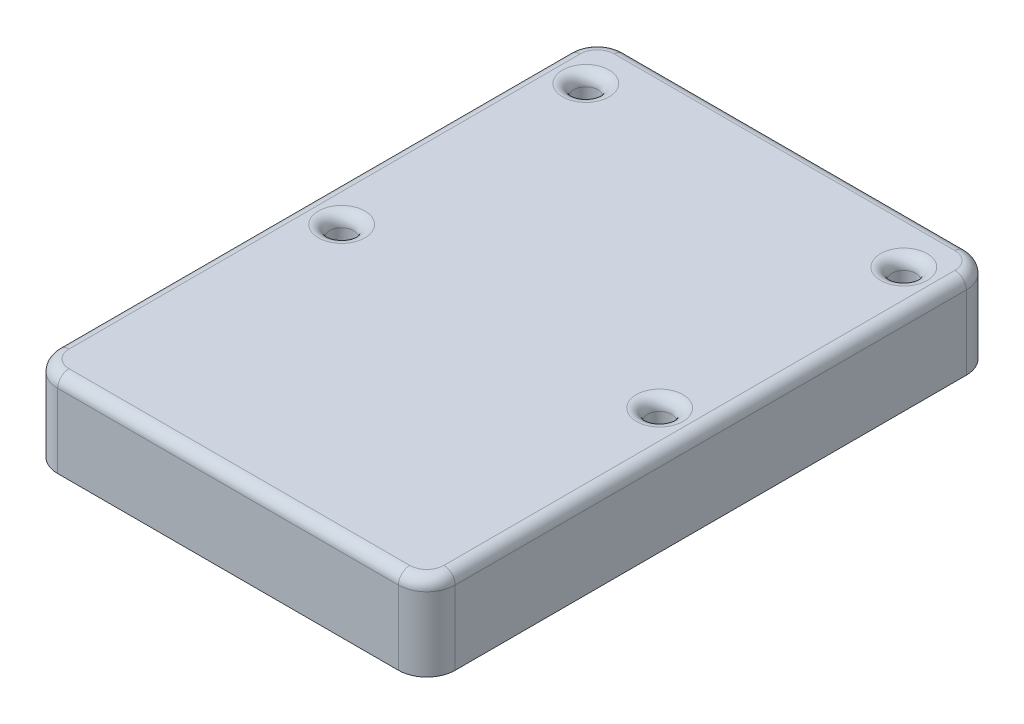
from build123d import *

# Parameters (mm, degrees)
BOSS_EXTRUDE1_DEPTH = 15
CUT_EXTRUDE1_DEPTH  = 12
CUT_EXTRUDE2_DEPTH  = 1
BOSS_EXTRUDE2_START = 11
BOSS_EXTRUDE2_DEPTH = 11
SKETCH5_R           = 1.2
CUT_EXTRUDE3_DEPTH  = 63.84902545
SKETCH6_R           = 2.1
CUT_EXTRUDE4_DEPTH  = 12
FILLET1_R           = 2
SCALE1_SCALE        = 0.5
FILLET2_R           = 1


with BuildPart() as part:
    # Sketch1 → Boss-Extrude1 (new body)
    with BuildSketch(Plane(origin=(0, 0, 0), x_dir=(1, 0, 0), z_dir=(0, 1, 0))):
        with BuildLine():
            Line((-30, -50), (30, -50))
            ThreePointArc((30, -50), (33.535533906, -48.535533906), (35, -45))
            Line((35, -45), (35, 45))
            ThreePointArc((35, 45), (33.535533906, 48.535533906), (30, 50))
            Line((30, 50), (-30, 50))
            ThreePointArc((-30, 50), (-33.535533906, 48.535533906), (-35, 45))
            Line((-35, 45), (-35, -45))
            ThreePointArc((-35, -45), (-33.535533906, -48.535533906), (-30, -50))
        make_face()
    extrude(amount=BOSS_EXTRUDE1_DEPTH)

    # Sketch2 → Cut-Extrude1 (cut)
    with BuildSketch(Plane.XZ):
        with BuildLine():
            Line((-27, -47), (27, -47))
            ThreePointArc((27, -47), (30.535533906, -45.535533906), (32, -42))
            Line((32, -42), (32, 42))
            ThreePointArc((32, 42), (30.535533906, 45.535533906), (27, 47))
            Line((27, 47), (-27, 47))
            ThreePointArc((-27, 47), (-30.535533906, 45.535533906), (-32, 42))
            Line((-32, 42), (-32, -42))
            ThreePointArc((-32, -42), (-30.535533906, -45.535533906), (-27, -47))
        make_face()
    extrude(amount=-CUT_EXTRUDE1_DEPTH, mode=Mode.SUBTRACT)

    # Sketch3 → Cut-Extrude2 (cut)
    with BuildSketch(Plane.XZ):
        with BuildLine():
            Line((-27, -48.55), (27, -48.55))
            ThreePointArc((27, -48.55), (31.631549417, -46.631549417), (33.55, -42))
            Line((33.55, -42), (33.55, 42))
            ThreePointArc((33.55, 42), (31.631549417, 46.631549417), (27, 48.55))
            Line((27, 48.55), (-27, 48.55))
            ThreePointArc((-27, 48.55), (-31.631549417, 46.631549417), (-33.55, 42))
            Line((-33.55, 42), (-33.55, -42))
            ThreePointArc((-33.55, -42), (-31.631549417, -46.631549417), (-27, -48.55))
        make_face()
        with BuildLine():
            Line((-27, -47), (27, -47))
            ThreePointArc((27, -47), (30.535533906, -45.535533906), (32, -42))
            Line((32, -42), (32, 42))
            ThreePointArc((32, 42), (30.535533906, 45.535533906), (27, 47))
            Line((27, 47), (-27, 47))
            ThreePointArc((-27, 47), (-30.535533906, 45.535533906), (-32, 42))
            Line((-32, 42), (-32, -42))
            ThreePointArc((-32, -42), (-30.535533906, -45.535533906), (-27, -47))
        make_face(mode=Mode.SUBTRACT)
    extrude(amount=-CUT_EXTRUDE2_DEPTH, mode=Mode.SUBTRACT)

    # Sketch4 → Boss-Extrude2 (add)
    with BuildSketch(Plane.XZ.offset(-12).offset(BOSS_EXTRUDE2_START)):
        with BuildLine():
            ThreePointArc((-28, -2), (-24, 2), (-28, 6))
            Line((-28, 6), (-32, 6))
            Line((-32, 6), (-32, -2))
            Line((-32, -2), (-28, -2))
        make_face()
        with BuildLine():
            Line((-28, -37), (-32, -37))
            Line((-32, -37), (-32, -42))
            ThreePointArc((-32, -42), (-30.535533906, -45.535533906), (-27, -47))
            Line((-27, -47), (-24, -47))
            Line((-24, -47), (-24, -41))
            ThreePointArc((-24, -41), (-25.171572875, -38.171572875), (-28, -37))
        make_face()
        with BuildLine():
            Line((32, -2), (32, 6))
            Line((32, 6), (28, 6))
            ThreePointArc((28, 6), (24, 2), (28, -2))
            Line((28, -2), (32, -2))
        make_face()
        with BuildLine():
            Line((24, -41), (24, -47))
            Line((24, -47), (27, -47))
            ThreePointArc((27, -47), (30.535533906, -45.535533906), (32, -42))
            Line((32, -42), (32, -37))
            Line((32, -37), (28, -37))
            ThreePointArc((28, -37), (25.171572875, -38.171572875), (24, -41))
        make_face()
    extrude(amount=-BOSS_EXTRUDE2_DEPTH)

    # Sketch5 → Cut-Extrude3 (cut, through all)
    with BuildSketch(Plane(origin=(0, 15, 0), x_dir=(1, 0, 0), z_dir=(0, 1, 0))):
        with Locations(Location((28, -2, 0), (0, 0, 270))):
            Circle(SKETCH5_R)
        with Locations(Location((28, 41, 0), (0, 0, 270))):
            Circle(SKETCH5_R)
        with Locations(Location((-28, 41, 0), (0, 0, 270))):
            Circle(SKETCH5_R)
        with Locations(Location((-28, -2, 0), (0, 0, 270))):
            Circle(SKETCH5_R)
    extrude(amount=-CUT_EXTRUDE3_DEPTH, mode=Mode.SUBTRACT)

    # Sketch6 → Cut-Extrude4 (cut)
    with BuildSketch(Plane(origin=(0, 15, 0), x_dir=(1, 0, 0), z_dir=(0, 1, 0))):
        with Locations(Location((28, -2, 0), (0, 0, 270))):
            Circle(SKETCH6_R)
        with Locations(Location((-28, -2, 0), (0, 0, 270))):
            Circle(SKETCH6_R)
        with Locations(Location((-28, 41, 0), (0, 0, 270))):
            Circle(SKETCH6_R)
        with Locations(Location((28, 41, 0), (0, 0, 270))):
            Circle(SKETCH6_R)
    extrude(amount=-CUT_EXTRUDE4_DEPTH, mode=Mode.SUBTRACT)

    # Fillet1
    fillet1_edges = [part.edges().sort_by_distance(p)[0] for p in [
        (33.535533906, 15, 48.535533906),
        (35, 15, 0),
        (33.535533906, 15, -48.535533906),
        (0, 15, -50),
        (28, 15, -43.1),
        (-28, 15, -43.1),
        (-28, 15, -0.1),
        (28, 15, -0.1),
        (-33.535533906, 15, -48.535533906),
        (-35, 15, 0),
        (-33.535533906, 15, 48.535533906),
        (0, 15, 50),
    ]]
    fillet(fillet1_edges, radius=FILLET1_R)


with BuildPart() as part_1:
    # Scale1: scaled about (0, 10.592691126, -1.421166574)
    add(part.part.scale(SCALE1_SCALE).moved(Location((0, 5.296345563, -0.710583287))))

    # Fillet2
    fillet2_edges = [part_1.edges().sort_by_distance(p)[0] for p in [
        (-16, 8.546345563, -1.710583287),
        (-16, 8.546345563, 2.289416713),
        (16, 8.546345563, 2.289416713),
        (16, 8.546345563, -1.710583287),
        (16, 8.546345563, -19.210583287),
        (12, 8.546345563, -24.210583287),
        (-12, 8.546345563, -24.210583287),
        (-16, 8.546345563, -19.210583287),
    ]]
    fillet(fillet2_edges, radius=FILLET2_R)


solid = part_1.part
